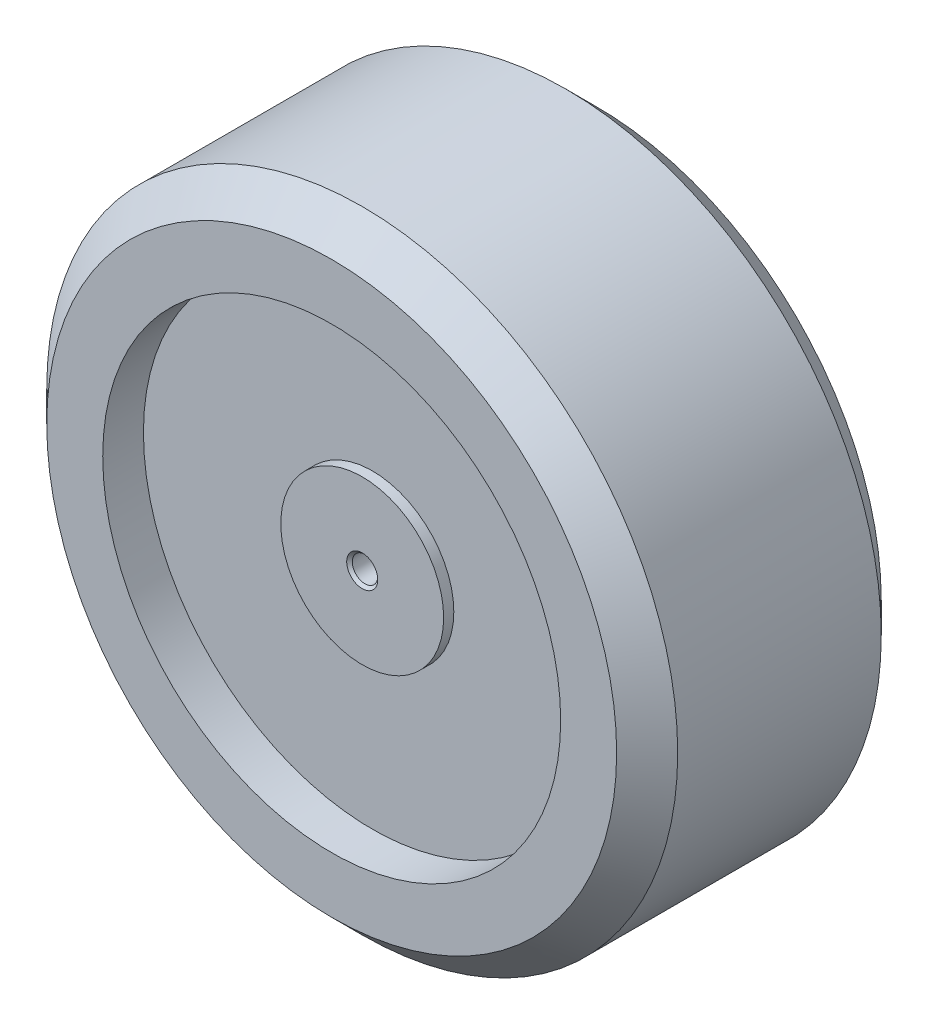
SolidWorks part; units mm, degrees
ref_plane "Front Plane" through (0, 0, 0) normal (0, 0, 1) x (1, 0, 0)
ref_plane "Top Plane" through (0, 0, 0) normal (0, 1, 0) x (1, 0, 0)
ref_plane "Right Plane" through (0, 0, 0) normal (1, 0, 0) x (0, 0, -1)
other "Configuration Table"
sketch "Sketch1" plane through (0, 0, 0) normal (0, 0, 1) x (1, 0, 0)
  circle A0 centre (0, 0) radius 31
  dimension "D1" = 62
extrude "Boss-Extrude1" add sketch "Sketch1" along normal blind 26
sketch "Sketch2" plane through (0, 0, 0) normal (0, 0, -1) x (-1, 0, 0)
  circle A0 centre (0, 0) radius 22.5
  dimension "D1" = 45
extrude "Cut-Extrude1" cut sketch "Sketch2" against normal blind 11
sketch "Sketch3" plane through (0, 0, 11) normal (0, 0, -1) x (-1, 0, 0)
  line L1 (0, 6.9282) -> (-6, 3.4641)
  line L2 (-6, 3.4641) -> (-6, -3.4641)
  line L3 (-6, -3.4641) -> (0, -6.9282)
  line L4 (0, -6.9282) -> (6, -3.4641)
  line L5 (6, -3.4641) -> (6, 3.4641)
  line L6 (6, 3.4641) -> (0, 6.9282)
  circle A0 centre (0, 0) radius 6 construction
  dimension "D1" = 12
extrude "Cut-Extrude2" cut sketch "Sketch3" against normal blind 3.1
sketch "Sketch4" plane through (0, 0, 26) normal (0, 0, 1) x (1, 0, 0)
  circle A0 centre (0, 0) radius 8
  circle A1 centre (0, 0) radius 22.5
  dimension "D1" = 16
  dimension "D2" = 45
extrude "Cut-Extrude3" cut sketch "Sketch4" against normal blind 4
sketch "Sketch5" plane through (0, 0, 26) normal (0, 0, 1) x (1, 0, 0)
  circle A1 centre (0, 0) radius 8
  circle A2 centre (0, 0) radius 8
  dimension "D1" = 0
extrude "Cut-Extrude4" cut sketch "Sketch5" against normal blind 3
hole_wizard "M3 Tapped Hole1" positions "Sketch7" profile "Sketch8" tap size "M3" standard "GB" end condition up to next
sketch "Sketch7" plane through (0, 0, 23) normal (0, 0, 1) x (1, 0, 0)
  point P0 (0, 0)
sketch "Sketch8" plane through (0, 0, 23) normal (1, 0, 0) x (0, -1, 0)
  line L0 (0, 0) -> (0, 8.9)
  line L1 (0, 8.9) -> (1.25, 8.9)
  line L2 (1.25, 8.9) -> (1.25, 0.275)
  line L3 (1.25, 0.275) -> (1.525, 0)
  line L5 (1.525, 0) -> (0, 0)
  line L6 (-1.25, 0.275) -> (-1.525, 0) construction
  line L11 (0, -6.35) -> (0, 107.95) construction
  dimension "通孔螺纹孔钻头直径" = 2.5
  dimension "通孔螺纹孔钻头深度" = 8.9
  dimension "近端锥形沉头孔直径" = 3.05
  dimension "近端锥形沉头孔角度" = 90
cosmetic thread "Cosmetic thread1" parameters "D2"=3
chamfer "Chamfer1" distance 3 angle 45 2 edges at (31, 0, 26) (31, 0, 0)
